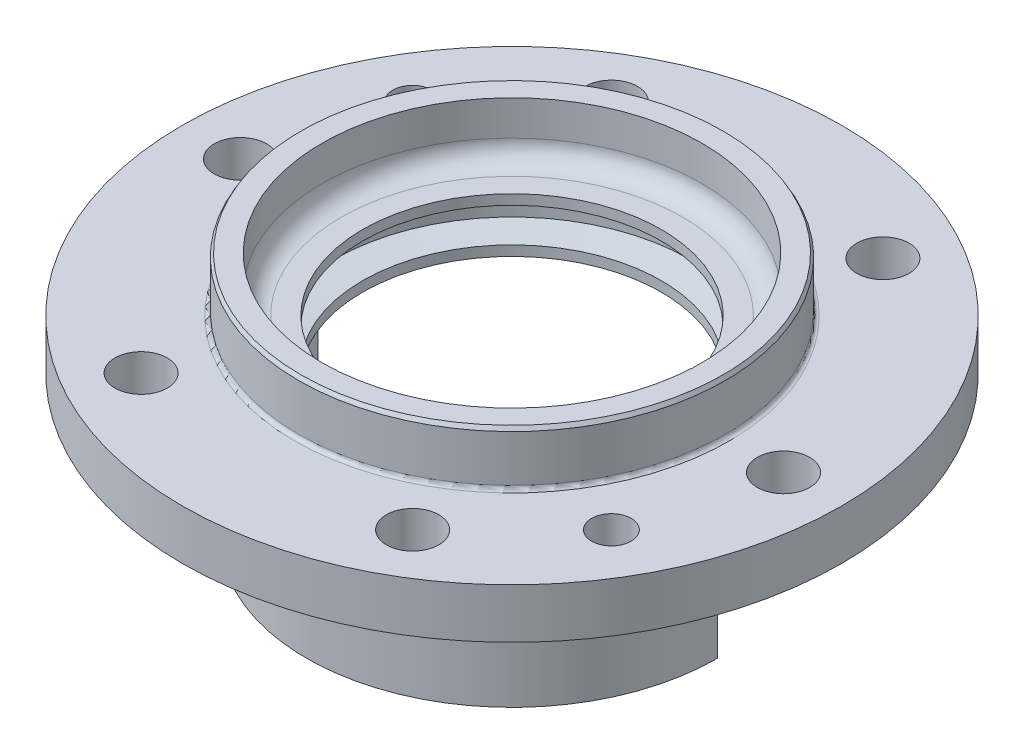
from build123d import *

# Parameters (mm, degrees)
SKETCH1_R           = 85
BOSS_EXTRUDE1_DEPTH = 14
SKETCH2_R           = 55
SKETCH2_R_2         = 49
BOSS_EXTRUDE2_DEPTH = 14
FILLET1_R           = 5
FILLET2_R           = 1
CHAMFER1_SIZE       = 2
CHAMFER1_SIZE2      = 1.154700538
CHAMFER2_SIZE       = 1
CHAMFER2_SIZE2      = 0.577350269
BOSS_EXTRUDE3_DEPTH = 36
SKETCH5_R           = 6.75
CUT_EXTRUDE1_DEPTH  = 126.483066587
CIRPATTERN1_COUNT   = 6
M12_TAPPED_HOLE1_D  = 10.2


with BuildPart() as part:
    # Sketch1 → Boss-Extrude1 (new body)
    with BuildSketch(Plane(origin=(0, 0, 0), x_dir=(1, 0, 0), z_dir=(0, 1, 0))):
        with Locations(Location((0, 0, 0), (0, 0, 270))):
            Circle(SKETCH1_R)
    extrude(amount=BOSS_EXTRUDE1_DEPTH)

    # Sketch2 → Boss-Extrude2 (add)
    with BuildSketch(Plane(origin=(0, 14, 0), x_dir=(1, 0, 0), z_dir=(0, 1, 0))):
        with Locations(Location((0, 0, 0), (0, 0, 270))):
            Circle(SKETCH2_R)
        with Locations(Location((0, 0, 0), (0, 0, 270))):
            Circle(SKETCH2_R_2, mode=Mode.SUBTRACT)
    extrude(amount=BOSS_EXTRUDE2_DEPTH)

    # Fillet1
    fillet1_edges = [part.edges().sort_by_distance(p)[0] for p in [
        (0, 14, -49),
    ]]
    fillet(fillet1_edges, radius=FILLET1_R)

    # Fillet2
    fillet2_edges = [part.edges().sort_by_distance(p)[0] for p in [
        (0, 14, -55),
    ]]
    fillet(fillet2_edges, radius=FILLET2_R)

    # Chamfer1
    chamfer1_edges = [part.edges().sort_by_distance(p)[0] for p in [
        (0, 0, -85),
    ]]
    chamfer1_side = [part.faces().sort_by_distance(p)[0] for p in [
        (0, 0, 0),
    ]]
    chamfer(chamfer1_edges, length=CHAMFER1_SIZE, length2=CHAMFER1_SIZE2, reference=chamfer1_side[0])

    # Chamfer2
    chamfer2_edges = [part.edges().sort_by_distance(p)[0] for p in [
        (0, 28, -55),
    ]]
    chamfer2_side = [part.faces().sort_by_distance(p)[0] for p in [
        (0, 21.5, -55),
    ]]
    chamfer(chamfer2_edges, length=CHAMFER2_SIZE, length2=CHAMFER2_SIZE2, reference=chamfer2_side[0])

    # Sketch3 → Boss-Extrude3 (add)
    with BuildSketch(Plane.XZ):
        with BuildLine():
            Line((-53, 0), (-50, 0))
            ThreePointArc((-50, 0), (0, 50), (50, 0))
            Line((50, 0), (53, 0))
            ThreePointArc((53, 0), (0, 53), (-53, 0))
        make_face()
    extrude(amount=BOSS_EXTRUDE3_DEPTH)

    # Sketch4 → Cut-Revolve1 (revolve, cut)
    with BuildSketch(Plane.XY):
        Polygon((-46, 10.5), (-46, 3.5), (-38.5, 2.579115793), (-38.5, 0), (0, 0), (0, 14), (-38.5, 14), (-38.5, 11.420884207), align=None)
    revolve(axis=Axis((0, 14, 0), (0, -1, 0)), mode=Mode.SUBTRACT)

    # Sketch5 → Cut-Extrude1 (cut, through all)
    with BuildSketch(Plane.XZ):
        with Locations(Location((-35, 60.621778265, 0), (0, 0, 270))):
            Circle(SKETCH5_R)
    cut_extrude1 = extrude(amount=-CUT_EXTRUDE1_DEPTH, mode=Mode.SUBTRACT)

    # CirPattern1: Cut-Extrude1 ×6 about axis
    cirpattern1_axis = Axis((0, 0, 0), (0, 1, 0))
    for i in range(1, CIRPATTERN1_COUNT):
        add(cut_extrude1.rotate(cirpattern1_axis, i * 360 / CIRPATTERN1_COUNT), mode=Mode.SUBTRACT)

    # M12 Tapped Hole1 (through all)
    with Locations(Plane(origin=(0, 0, 0), x_dir=(-1, 0, 0), z_dir=(0, -1, 0))):
        with Locations((-60.621778265, -35), (60.621778265, 35)):
            Hole(M12_TAPPED_HOLE1_D / 2)


solid = part.part
